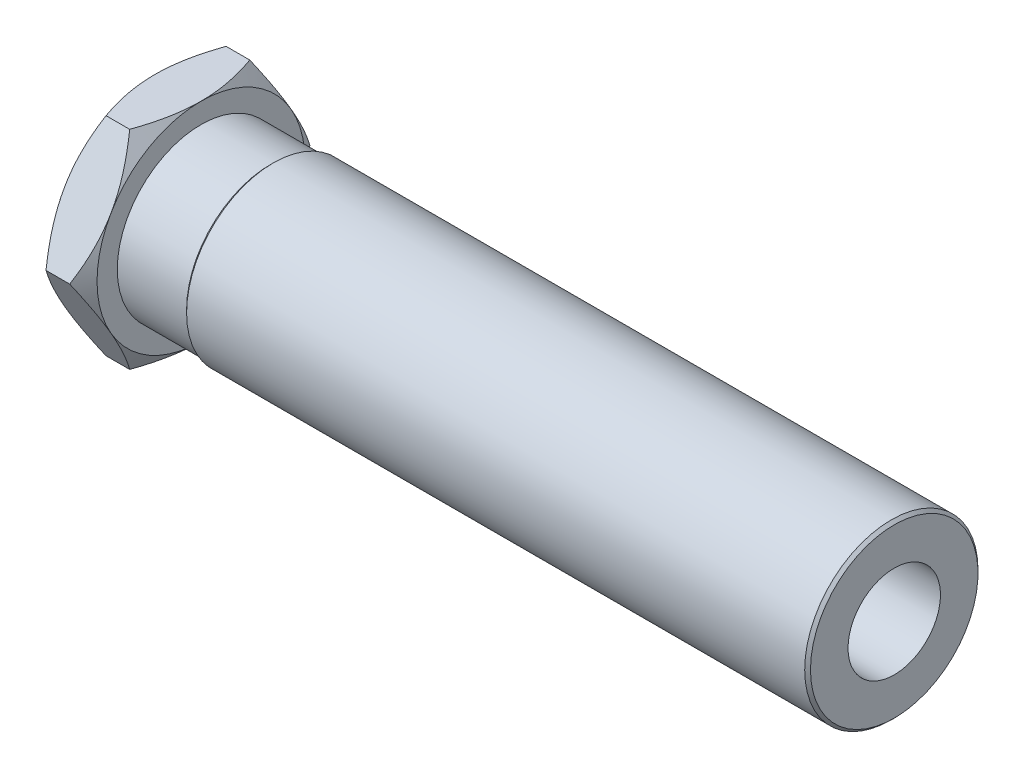
from build123d import *

# Parameters (mm, degrees)
EXTRUDE_714_DEPTH      = 8
SKETCH_2_2_R           = 23.58
SKETCH_2_2_R_2         = 18
CUT_EXTRUDE_1047_DEPTH = 8
CUT_EXTRUDE_1047_DRAFT = -55
SKETCH_5_R             = 23.569219382
SKETCH_5_R_2           = 18
CUT_EXTRUDE_2_DEPTH    = 6.0502
CUT_EXTRUDE_2_DRAFT    = -55


with BuildPart() as part:
    # Sketch 2 → 旋转1 (revolve)
    with BuildSketch(Plane.XY, mode=Mode.PRIVATE) as revolve_1_sk:
        Polygon((0, 0), (120, 0), (120, 14.5), (119.5, 15), (12.5, 15), (12, 14.5), (0, 14.5), align=None)
    revolve(revolve_1_sk.sketch.rotate(Axis((0, 0, 0), (1, 0, 0)), 90), axis=Axis((0, 0, 0), (1, 0, 0)))

    # Sketch 1 → Extrude 714 (add)
    with BuildSketch(Plane(origin=(0, -0.910076524, 0.397317176), x_dir=(0, 0, 1), z_dir=(-1, 0, 0))):
        Polygon((-21.181926867, 0.910076524), (-10.789622021, -17.089923476), (9.99498767, -17.089923476), (20.387292515, 0.910076524), (9.99498767, 18.910076524), (-10.789622021, 18.910076524), align=None)
    extrude(amount=EXTRUDE_714_DEPTH)


with BuildPart() as cut_extrude_1047_tool:
    # Sketch 2 2 → Cut-Extrude 1047 (with draft: the straight prism first)
    with BuildSketch(Plane.ZY.offset(8)):
        Circle(SKETCH_2_2_R)
        Circle(SKETCH_2_2_R_2, mode=Mode.SUBTRACT)
    extrude(amount=-CUT_EXTRUDE_1047_DEPTH)
    # Cut-Extrude 1047: the draft: its side faces are tilted about the plane it starts from
    cut_extrude_1047_sides = [cut_extrude_1047_tool.faces().sort_by_distance(p)[0] for p in [
        (-4, 0, -23.58),
        (-4, 0, -18),
    ]]
    draft(cut_extrude_1047_sides, Plane.ZY.offset(8), CUT_EXTRUDE_1047_DRAFT)


with BuildPart() as part_1:
    add(part.part)

    # Cut-Extrude 1047: cut by cut_extrude_1047_tool
    add(cut_extrude_1047_tool.part, mode=Mode.SUBTRACT)


with BuildPart() as cut_extrude_2_tool:
    # 草图5 → 切除-拉伸2 (with draft: the straight prism first)
    with BuildSketch(Plane(origin=(0, 0, 0), x_dir=(0, 0, -1), z_dir=(1, 0, 0))):
        Circle(SKETCH_5_R)
        Circle(SKETCH_5_R_2, mode=Mode.SUBTRACT)
    extrude(amount=-CUT_EXTRUDE_2_DEPTH)
    # 切除-拉伸2: the draft: its side faces are tilted about the plane it starts from
    cut_extrude_2_sides = [cut_extrude_2_tool.faces().sort_by_distance(p)[0] for p in [
        (-3.0251, 0, 23.569219382),
        (-3.0251, 0, 18),
    ]]
    draft(cut_extrude_2_sides, Plane(origin=(0, 0, 0), x_dir=(0, 0, -1), z_dir=(1, 0, 0)), CUT_EXTRUDE_2_DRAFT)


with BuildPart() as part_2:
    add(part_1.part)

    # 切除-拉伸2: cut by cut_extrude_2_tool
    add(cut_extrude_2_tool.part, mode=Mode.SUBTRACT)

    # 草图6 → 切除-旋转1 (revolve, cut)
    with BuildSketch(Plane.XY, mode=Mode.PRIVATE) as cut_revolve_1_sk:
        Polygon((0, 0), (120, 0), (120, 8), (-8, 8), (-8, 0), align=None)
    revolve(cut_revolve_1_sk.sketch.rotate(Axis((0, 0, 0), (1, 0, 0)), 90), axis=Axis((0, 0, 0), (1, 0, 0)), mode=Mode.SUBTRACT)


solid = part_2.part
